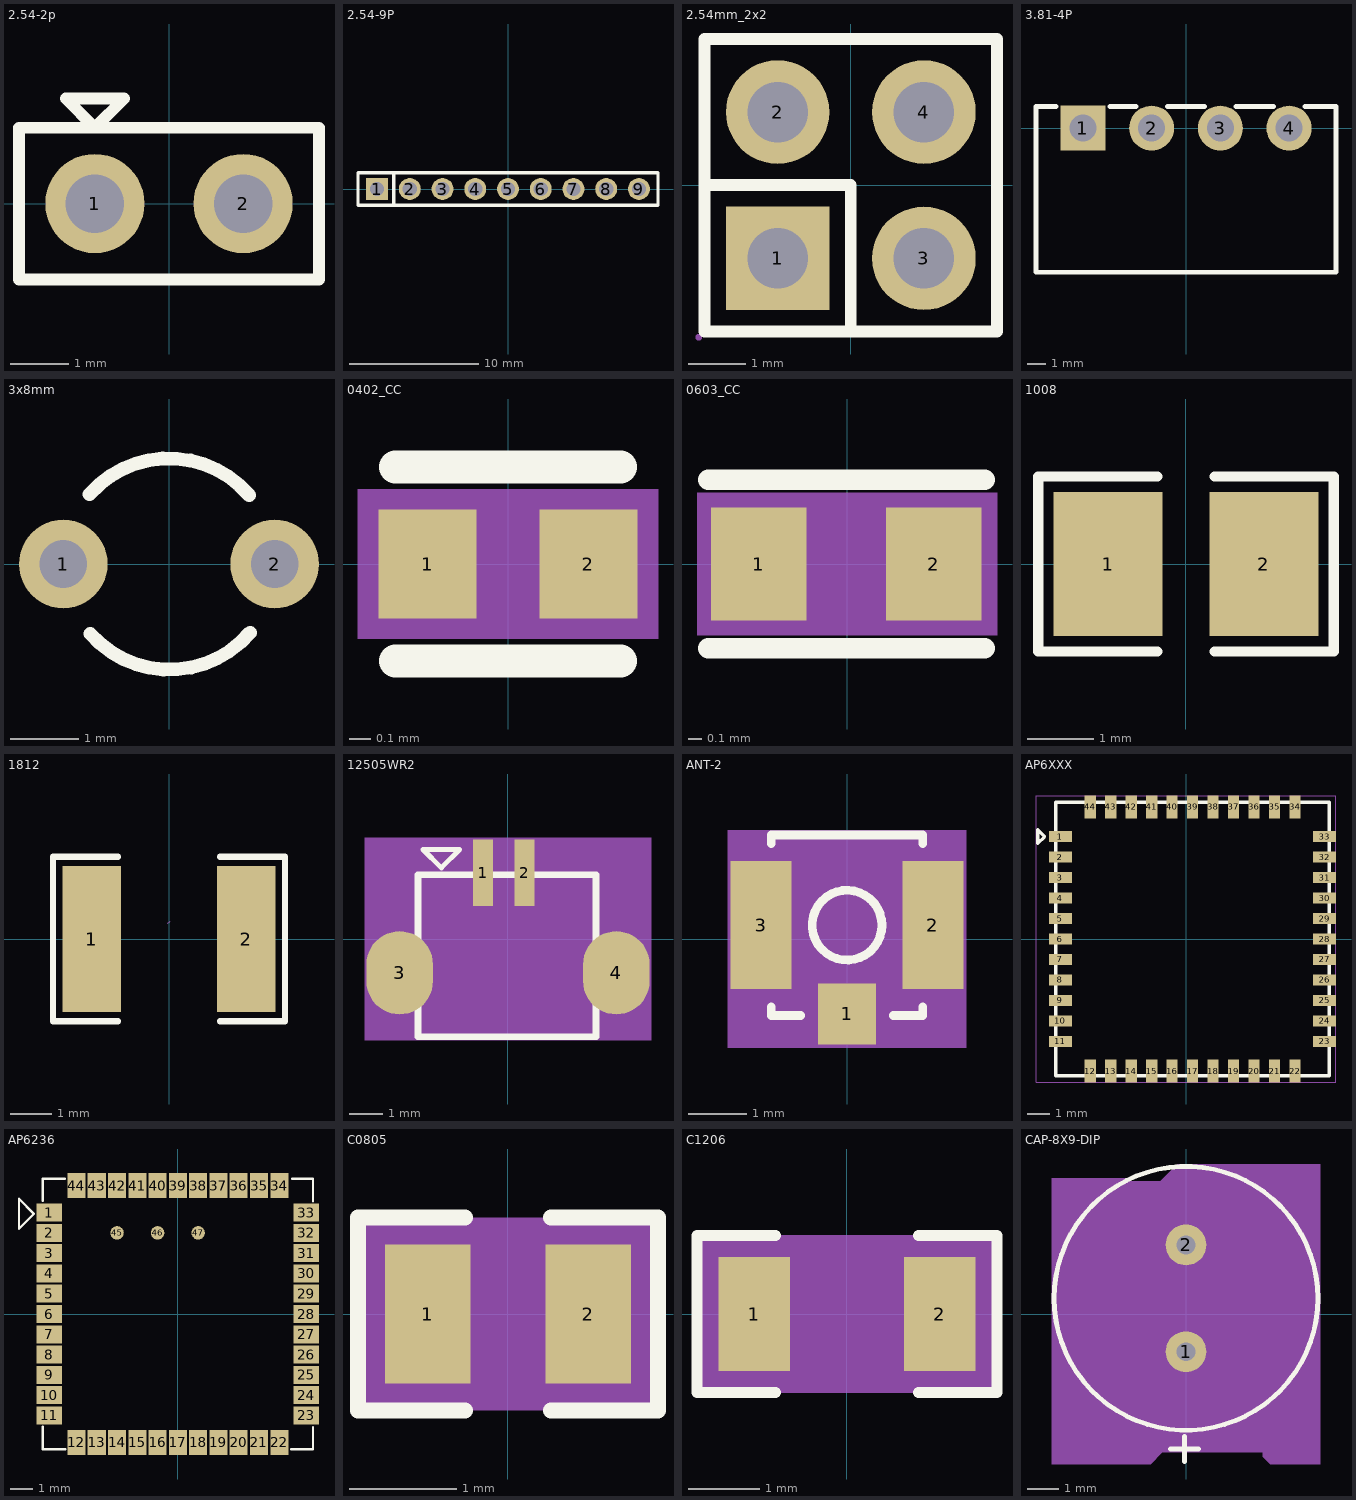
[diagram p0: the footprints below, top view; thin cyan lines are the x and y axes]
# Altium footprint library MISC84456-5.PcbLib: 85 footprints (part 1 of 6)
Each footprint in its own frame and in the unit in brackets; x right, y up, seen from the top. Pads: shape width x height; smd on the part's side, far side on the other; paste and mask are expansions set on the pad; w line width, h text height; cw(c..) or ccw(c..) is an arc to the next point about the centre after c.

## 2.54-2p [mm]
pads (2):
  round 1.7 hole 1: 1(-1.27,0) 2(1.27,0)
Top Overlay:
  lines w0.2: -2.57,0 -2.57,1.3 2.57,1.3 2.57,-1.3 -2.57,-1.3 -2.57,0.1 ; -1.77,1.8 -1.27,1.3 -0.77,1.8 -1.77,1.8
Mechanical 7:
  text "2" at 1.27,-0.254 h0.64
  text "1" at -1.27,-0.254 h0.64

## 2.54-9P [mm]
pads (9):
  rect 1.7x1.7 hole 1.1: 1(-10.16,0)
  round 1.7 hole 1.1: 2(-7.62,0) 3(-5.08,0) 4(-2.54,0) 5(0,0) 6(2.54,0) 7(5.08,0) 8(7.62,0) 9(10.16,0)
Top Overlay:
  lines w0.254: -8.866,-1.27 -8.866,1.27 ; -11.64,-1.27 11.64,-1.27 11.64,1.27 -11.64,1.27 -11.64,-1.27
Mechanical 15:
  lines w0.003: -0.025,0.451 0.025,0.502

## 2.54mm_2x2 [mm]
pads (4):
  rect 1.8x1.8 hole 1.05: 1(-1.27,-1.27)
  round 1.8 hole 1.05: 2(-1.27,1.27) 3(1.27,-1.27) 4(1.27,1.27)
Top Overlay:
  lines w0.203: -2.54,0.002 0,0.002 0,-2.54 ; 0.212,-2.54 2.54,-2.54 ; 2.54,-2.54 2.54,2.54 -2.54,2.54 -2.54,-2.54 2.54,-2.54
Mechanical 5:
  circle w0.425: c1.27,1.27 r0.213
  circle w0.425: c1.27,-1.27 r0.213
  circle w0.425: c-1.27,1.27 r0.213
  circle w0.425: c-1.27,-1.27 r0.213
Mechanical 6:
  circle w0.06: c-2.642,-2.642 r0.03

## 3.81-4P [mm]
pads (4):
  rect 2.5x2.5 hole 1.5: 1(-5.715,0)
  round 2.5 hole 1.5: 2(-1.905,0) 3(1.905,0) 4(5.715,0)
Top Overlay:
  lines w0.254: -7.196,1.2 -8.315,1.2 -8.315,-8 8.315,-8 8.315,1.2 6.581,1.2 ; -4.234,1.2 -2.771,1.2 ; -1.039,1.2 1.039,1.2 ; 2.771,1.2 4.849,1.2

## 3x8mm [mm]
pads (2):
  round 1.3 hole 0.7: 1(-1.55,0) 2(1.55,0)
Top Overlay:
  lines w0.2: -1.165,1.022 cw(c0,0) 1.179,1.006 ; -1.155,-1.022 ccw(c0.01,0) 1.189,-1.006

## 0402_CC [mil] "0402_CC"
pads (2):
  rect 18x20 smd: 1(-14.76,0) 2(14.76,0)
Top Overlay:
  lines w6: -20.67,-17.83 20.67,-17.83 ; -20.67,17.83 20.67,17.83
  text ".Designator" at 4.92,-164.76 h23.62
Mechanical 7:
  text "2" at 14.76,-4.72 h11.81
  text "1" at -14.76,-4.72 h11.81
Mechanical 8:
  region: -27.56,13.78 -27.56,-13.78 27.56,-13.78 27.56,13.78
Mechanical 9:
  text "0.1uF" at -31.5,-8.86 h13.78

## 0603_CC [mil] "0603_CC"
pads (2):
  rect 28x33 smd: 1(-25.79,0) 2(25.39,0)
Top Overlay:
  lines w6: -40.67,-24.72 40.27,-24.72 ; -40.67,24.72 40.27,24.72
Mechanical 7:
  text "1" at -25.79,-4.72 h11.81
  text "2" at 25.39,-4.72 h11.81
Mechanical 8:
  region: -38.78,-20.87 43.9,-20.87 43.9,20.87 -43.9,20.87 -43.9,-18.5 -43.9,-20.87
Mechanical 9:
  text ".Designator" at 1.77,-28.94 h13.78
  text "22uF" at -29.72,-3.94 h13.78

## 1008 [mm]
pads (2):
  rect 1.635x2.16 smd: 1(-1.168,0) 2(1.168,0)
Top Overlay:
  lines w0.152: -0.426,-1.309 -2.214,-1.309 -2.214,1.309 -0.426,1.309 ; 0.426,-1.309 2.214,-1.309 2.214,1.309 0.426,1.309
Top Paste:
  region: 0.315,-0.98 0.315,-0.467 0.415,-0.367 0.806,-0.367 0.906,-0.267 0.906,0.267 0.806,0.367 0.415,0.367 0.315,0.467 0.315,0.98 0.415,1.08 1.885,1.08 1.985,0.98 1.985,-0.98 1.885,-1.08 0.415,-1.08
  region: -0.315,-0.98 -0.315,-0.467 -0.415,-0.367 -0.806,-0.367 -0.906,-0.267 -0.906,0.267 -0.806,0.367 -0.415,0.367 -0.315,0.467 -0.315,0.98 -0.415,1.08 -1.885,1.08 -1.985,0.98 -1.985,-0.98 -1.885,-1.08 -0.415,-1.08

## 1812 [mm]
pads (2):
  rect 1.407x3.499 smd: 1(-1.853,0) 2(1.853,0)
Top Overlay:
  lines w0.152: -1.226,-1.978 -2.785,-1.978 -2.785,1.978 -1.226,1.978 ; 1.226,-1.978 2.785,-1.978 2.785,1.978 1.226,1.978
Top Paste:
  region: 1.15,-1.65 1.15,-0.695 1.25,-0.595 1.528,-0.595 1.628,-0.495 1.628,0.495 1.528,0.595 1.25,0.595 1.15,0.695 1.15,1.65 1.25,1.75 2.457,1.75 2.557,1.65 2.557,-1.65 2.457,-1.75 1.25,-1.75
  region: -1.15,-1.65 -1.15,-0.695 -1.25,-0.595 -1.528,-0.595 -1.628,-0.495 -1.628,0.495 -1.528,0.595 -1.25,0.595 -1.15,0.695 -1.15,1.65 -1.25,1.75 -2.457,1.75 -2.557,1.65 -2.557,-1.65 -2.457,-1.75 -1.25,-1.75
Mechanical 5:
  region: -2.275,-1.62 -2.275,1.62 -1.525,1.62 -1.525,-1.62
  region: 2.275,-1.62 2.275,1.62 1.525,1.62 1.525,-1.62
Mechanical 6:
  circle w0.06: c-2.275,-1.62 r0.03
Mechanical 15:
  lines w0.003: -0.025,0.376 0.025,0.427

## 12505WR2 [mm] "12505WR2"
pads (4):
  rect 0.6x2 smd: 1(-0.75,1.986) 2(0.5,1.986)
  oval 2x2.5 smd: 3(-3.25,-1.014) 4(3.25,-1.014)
Top Overlay:
  lines w0.152: -2.55,2.686 -2,2.136 -1.45,2.686 -2.55,2.686
  lines w0.203: -2.7,-2.934 2.64,-2.934 2.64,1.926 -2.7,1.926 -2.7,-2.934
Mechanical 7:
  text "1" at -0.496,1.986 h0.64
  text "2" at 0.754,1.986 h0.64
  text "4" at 3.504,-1.014 h0.64
  text "3" at -2.996,-1.014 h0.64
Mechanical 8:
  region: -4.3,-3.036 4.3,-3.036 4.3,3.036 -4.3,3.036
Mechanical 9:
  text "3V" at 0.65,-1.964 h0.35
  text ".Designator" at 0.75,-1.889 h0.35

## ANT-2 [mm] "ANT-2"
pads (3):
  rect 1.001x1.049 smd: 1(0,-1.286)
  rect 1.049x2.2 smd: 2(1.476,0.238) 3(-1.476,0.238)
Top Overlay:
  circle w0.15: c0,0.238 r0.599
  lines w0.15: -1.301,-1.162 -1.301,-1.312 -0.8,-1.312 ; -1.301,1.637 -1.301,1.787 1.301,1.787 1.301,1.637 ; 0.8,-1.312 1.301,-1.312 1.301,-1.162
  text ".Designator" at 2.75,1.313 h0.6
Mechanical 7:
  text "2" at 1.476,0.492 h0.64
  text "3" at -1.476,0.492 h0.64
  text "1" at 0,-1.032 h0.64
Mechanical 8:
  region: -2.05,-1.863 2.05,-1.863 2.05,1.863 -2.05,1.863
Mechanical 9:
  text "RF_3P" at -0.175,1.413 h0.35

## AP6XXX [mm] "AP6XXX"
pads (44):
  rect 1x0.5 smd: 1(-5.513,4.5) 2(-5.513,3.6) 3(-5.513,2.7) 4(-5.513,1.8) 5(-5.513,0.9) 6(-5.513,0) 7(-5.513,-0.9) 8(-5.513,-1.8) 9(-5.513,-2.7) 10(-5.513,-3.6) 11(-5.513,-4.5) 23(6.087,-4.5) 24(6.087,-3.6) 25(6.087,-2.7) 26(6.087,-1.8) 27(6.087,-0.9) 28(6.087,0) 29(6.087,0.9) 30(6.087,1.8) 31(6.087,2.7) 32(6.087,3.6) 33(6.087,4.5)
  rect 0.5x1 smd: 12(-4.213,-5.8) 13(-3.313,-5.8) 14(-2.413,-5.8) 15(-1.513,-5.8) 16(-0.613,-5.8) 17(0.288,-5.8) 18(1.187,-5.8) 19(2.087,-5.8) 20(2.987,-5.8) 21(3.887,-5.8) 22(4.787,-5.8) 34(4.787,5.8) 35(3.887,5.8) 36(2.987,5.8) 37(2.087,5.8) 38(1.187,5.8) 39(0.288,5.8) 40(-0.613,5.8) 41(-1.513,5.8) 42(-2.413,5.8) 43(-3.313,5.8) 44(-4.213,5.8)
Top Overlay:
  lines w0.15: -6.513,4.2 -6.513,4.8 -6.213,4.5 -6.513,4.2 ; -5.713,-6 6.287,-6 6.287,6 -5.713,6 -5.713,-6
  text ".Designator" at -0.138,8.175 h0.6
Mechanical 7:
  text "7" at -5.716,-0.9 h0.51
  text "13" at -3.719,-5.8 h0.51
  text "6" at -5.716,0 h0.51
  text "14" at -2.819,-5.8 h0.51
  text "2" at -5.716,3.6 h0.51
  text "10" at -5.919,-3.6 h0.51
  text "16" at -1.019,-5.8 h0.51
  text "29" at 5.681,0.9 h0.51
  text "22" at 4.381,-5.8 h0.51
  text "43" at -3.719,5.8 h0.51
  text "9" at -5.716,-2.7 h0.51
  text "19" at 1.681,-5.8 h0.51
  text "21" at 3.481,-5.8 h0.51
  text "42" at -2.819,5.8 h0.51
  text "15" at -1.919,-5.8 h0.51
  text "23" at 5.681,-4.5 h0.51
  text "41" at -1.919,5.8 h0.51
  text "44" at -4.619,5.8 h0.51
  text "12" at -4.619,-5.8 h0.51
  text "24" at 5.681,-3.6 h0.51
  text "18" at 0.781,-5.8 h0.51
  text "11" at -5.919,-4.5 h0.51
  text "34" at 4.381,5.8 h0.51
  text "17" at -0.119,-5.8 h0.51
  text "8" at -5.716,-1.8 h0.51
  text "4" at -5.716,1.8 h0.51
  text "32" at 5.681,3.6 h0.51
  text "37" at 1.681,5.8 h0.51
  text "35" at 3.481,5.8 h0.51
  text "38" at 0.781,5.8 h0.51
  text "5" at -5.716,0.9 h0.51
  text "26" at 5.681,-1.8 h0.51
  text "27" at 5.681,-0.9 h0.51
  text "25" at 5.681,-2.7 h0.51
  text "28" at 5.681,0 h0.51
  text "30" at 5.681,1.8 h0.51
  text "40" at -1.019,5.8 h0.51
  text "39" at -0.119,5.8 h0.51
  text "20" at 2.581,-5.8 h0.51
  text "31" at 5.681,2.7 h0.51
  text "33" at 5.681,4.5 h0.51
  text "1" at -5.716,4.5 h0.51
  text "3" at -5.716,2.7 h0.51
  text "36" at 2.581,5.8 h0.51
Mechanical 8:
  lines w0.025: -6.588,-6.3 6.587,-6.3 6.587,6.3 -6.588,6.3 -6.588,-6.3
Mechanical 9:
  text "AP6236" at -1.188,3.675 h0.35

## AP6236 [mm]
pads (47):
  rect 1.125x0.8 smd: 1(-5.7,4.5) 2(-5.7,3.6) 3(-5.7,2.7) 4(-5.7,1.8) 5(-5.7,0.9) 6(-5.7,0) 7(-5.7,-0.9) 8(-5.7,-1.8) 9(-5.7,-2.7) 10(-5.7,-3.6) 11(-5.7,-4.5) 23(5.7,-4.5) 24(5.7,-3.6) 25(5.7,-2.7) 26(5.7,-1.8) 27(5.7,-0.9) 28(5.7,0) 29(5.7,0.9) 30(5.7,1.8) 31(5.7,2.7) 32(5.7,3.6) 33(5.7,4.5)
  rect 0.8x1.125 smd: 12(-4.5,-5.7) 13(-3.6,-5.7) 14(-2.7,-5.7) 15(-1.8,-5.7) 16(-0.9,-5.7) 17(0,-5.7) 18(0.9,-5.7) 19(1.8,-5.7) 20(2.7,-5.7) 21(3.6,-5.7) 22(4.5,-5.7) 34(4.5,5.7) 35(3.6,5.7) 36(2.7,5.7) 37(1.8,5.7) 38(0.9,5.7) 39(0,5.7) 40(-0.9,5.7) 41(-1.8,5.7) 42(-2.7,5.7) 43(-3.6,5.7) 44(-4.5,5.7)
  round 0.6 smd: 45(-2.7,3.6) 46(-0.9,3.6) 47(0.9,3.6)
Top Overlay:
  lines w0.1: -6,-5 -6,-6 -4.99,-6 ; -6,5.01 -6,6 -5.02,6 ; 5.02,-6 6,-6 6,-5.01 ; 5.07,6 6,6 6,4.99 ; -6.38,4.44 -6.39,4.44 -7.05,3.78 -7.05,5.11 -6.38,4.44 ; -6.38,4.44 -6.38,4.44

## C0805 [mm] "C0805"
pads (2):
  rect 0.8x1.3 smd: 1(-0.75,0) 2(0.75,0)
Top Overlay:
  lines w0.15: -0.4,-0.9 -1.4,-0.9 -1.4,0.9 -0.4,0.9 ; 0.4,-0.9 1.4,-0.9 1.4,0.9 0.4,0.9
  text ".Designator" at 1.8,0.95 h0.6
Mechanical 7:
  text "1" at -0.75,0.254 h0.64
  text "2" at 0.75,0.254 h0.64
Mechanical 8:
  region: 1.4,0.9 -1.4,0.9 -1.4,-0.9 1.4,-0.9
Mechanical 9:
  text "PZ2012U221-2R0TF" at 2.9,0.025 h0.35

## C1206 [mm] "C1206"
pads (2):
  rect 1x1.6 smd: 1(-1.299,0) 2(1.3,0)
Top Overlay:
  lines w0.15: -1,-1.1 -2.1,-1.1 -2.1,1.1 -1,1.1 ; 1,-1.1 2.1,-1.1 2.1,1.1 1,1.1
Mechanical 7:
  text "2" at 1.554,0 h0.64
  text "1" at -1.045,0 h0.64
Mechanical 8:
  region: 2.1,-1.1 2.1,1.1 -2.1,1.1 -2.1,-1.1
Mechanical 9:
  text "1000pF-2KV" at 1.875,0.1 h0.35
  text ".Designator" at 0.825,0.325 h0.35

## CAP-8X9-DIP [mm] "CAP-8X9-DIP"
pads (2):
  round 1.3 hole 0.6: 1(0,-1.2) 2(0,2.2)
Top Overlay:
  circle w0.15: c0,0.5 r4.2
  lines w0.15: -0.5,-4.3 0.4,-4.3 ; -0.05,-4.7 -0.05,-3.9
  text ".Designator" at -5.15,0.85 h0.6
Mechanical 7:
  text "1" at -0.254,-1.2 h0.64
  text "2" at -0.254,2.2 h0.64
Mechanical 8:
  region: -4.275,-4.775 -1.125,-4.775 -0.75,-4.4 2.45,-4.4 2.45,-4.55 2.675,-4.775 4.275,-4.775 4.275,4.775 -0.275,4.775 -0.825,4.225 -1.725,4.225 -1.825,4.325 -4.275,4.325
Mechanical 9:
  text "470uF16V" at -1.7,0.15 h0.35